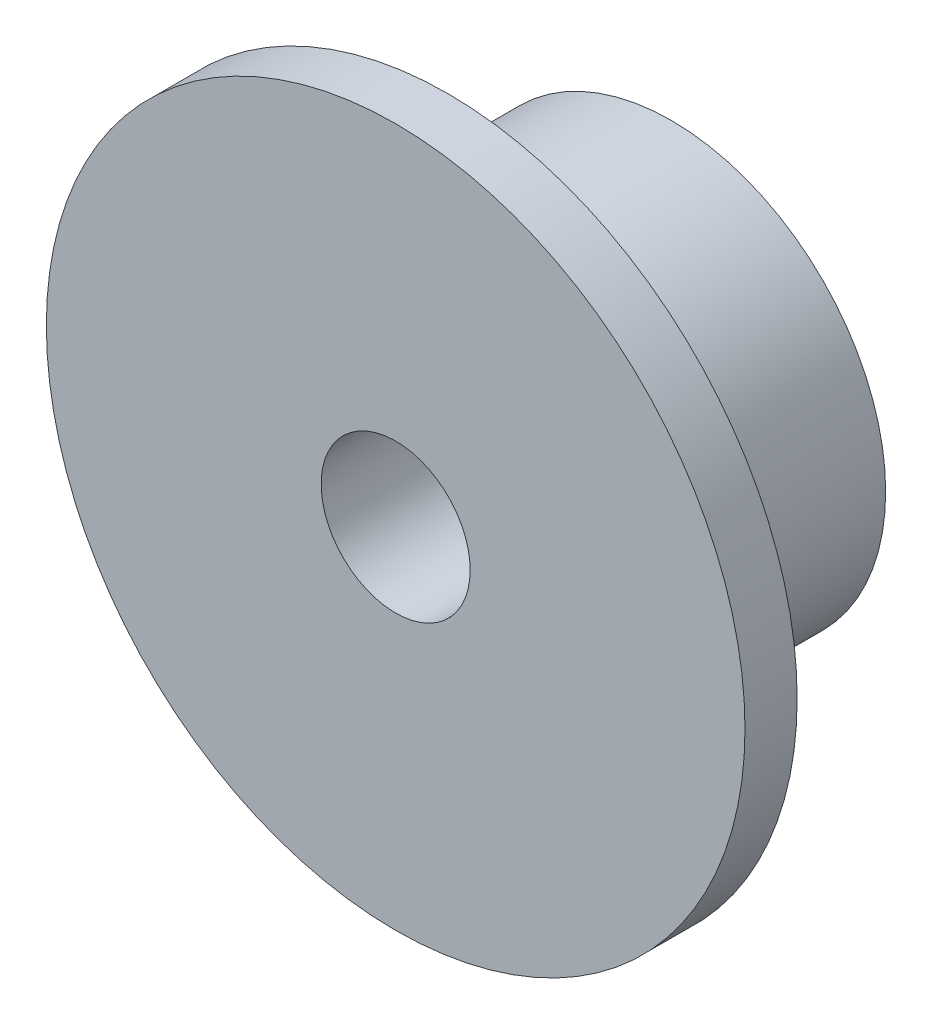
SolidWorks part; units mm, degrees
ref_plane "前视基准面" through (0, 0, 0) normal (0, 0, 1) x (1, 0, 0)
ref_plane "上视基准面" through (0, 0, 0) normal (0, 1, 0) x (1, 0, 0)
ref_plane "右视基准面" through (0, 0, 0) normal (1, 0, 0) x (0, 0, -1)
sketch "草图1" plane through (0, 0, 0) normal (0, 0, 1) x (1, 0, 0)
  circle A0 centre (0, 0) radius 4
  circle A1 centre (0, 0) radius 11.5
  dimension "D1" = 8
  dimension "D2" = 23
extrude "凸台-拉伸1" add sketch "草图1" along normal blind 12
sketch "草图2" plane through (0, 0, 12) normal (0, 0, 1) x (1, 0, 0)
  circle A0 centre (0, 0) radius 4
  circle A1 centre (0, 0) radius 18.75
  dimension "D1" = 37.5
  dimension "D2" = 8
extrude "凸台-拉伸2" add sketch "草图2" along normal blind 2.8
